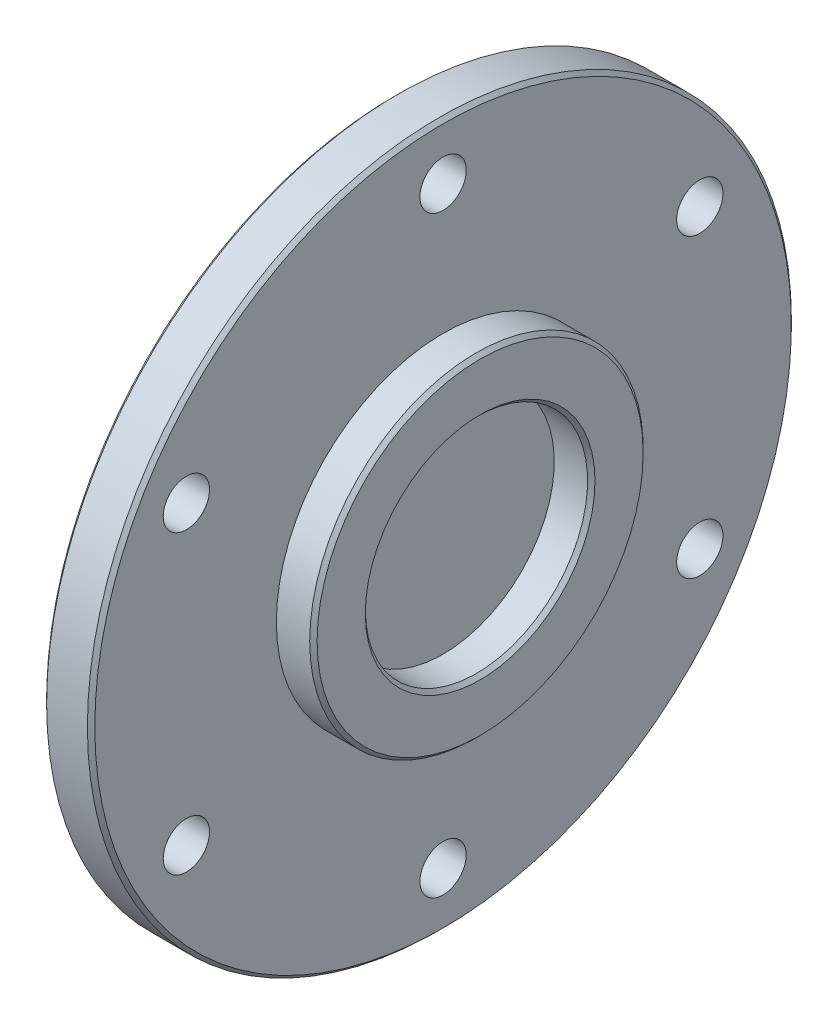
SolidWorks part; units mm, degrees
material "普通碳钢"
ref_plane "前视基准面" through (0, 0, 0) normal (0, 0, 1) x (1, 0, 0)
ref_plane "上视基准面" through (0, 0, 0) normal (0, 1, 0) x (1, 0, 0)
ref_plane "右视基准面" through (0, 0, 0) normal (1, 0, 0) x (0, 0, -1)
sketch "草图1" plane through (0, 0, 0) normal (0, 0, 1) x (1, 0, 0)
  line L0 (0, 0) -> (0, 290.7532) construction
  line L1 (0, 0) -> (356.4696, 0) construction
  line L2 (0, 0) -> (0, 95)
  line L3 (0, 95) -> (13, 95)
  line L4 (13, 95) -> (13, 45)
  line L5 (13, 45) -> (23, 45)
  line L6 (23, 45) -> (23, 30)
  line L7 (23, 30) -> (13, 30)
  line L8 (13, 30) -> (13, 0)
  line L9 (13, 0) -> (0, 0)
  dimension "D1" = 190
  dimension "D2" = 90
  dimension "D3" = 15
  dimension "D4" = 13
  dimension "D5" = 10
revolve "旋转1" add sketch "草图1" angle 360 about L1
sketch "草图2" plane through (0, 0, 0) normal (-1, 0, 0) x (0, 0, 1)
  line L0 (0, 0) -> (0, 80) construction
  circle A0 centre (0, 80) radius 6.25
  dimension "D2" = 12.5
  dimension "D1" = 80
extrude "切除-拉伸1" cut sketch "草图2" against normal through all
pattern_circular "阵列(圆周)1" count 6 over 360 about axis through (0, 0, 0) along (1, 0, 0) of "切除-拉伸1"
chamfer "倒角1" distance 1 angle 45 4 edges at (23, 0, 30) (23, 0, 45) (0, 0, 95) (13, 0, 95)
